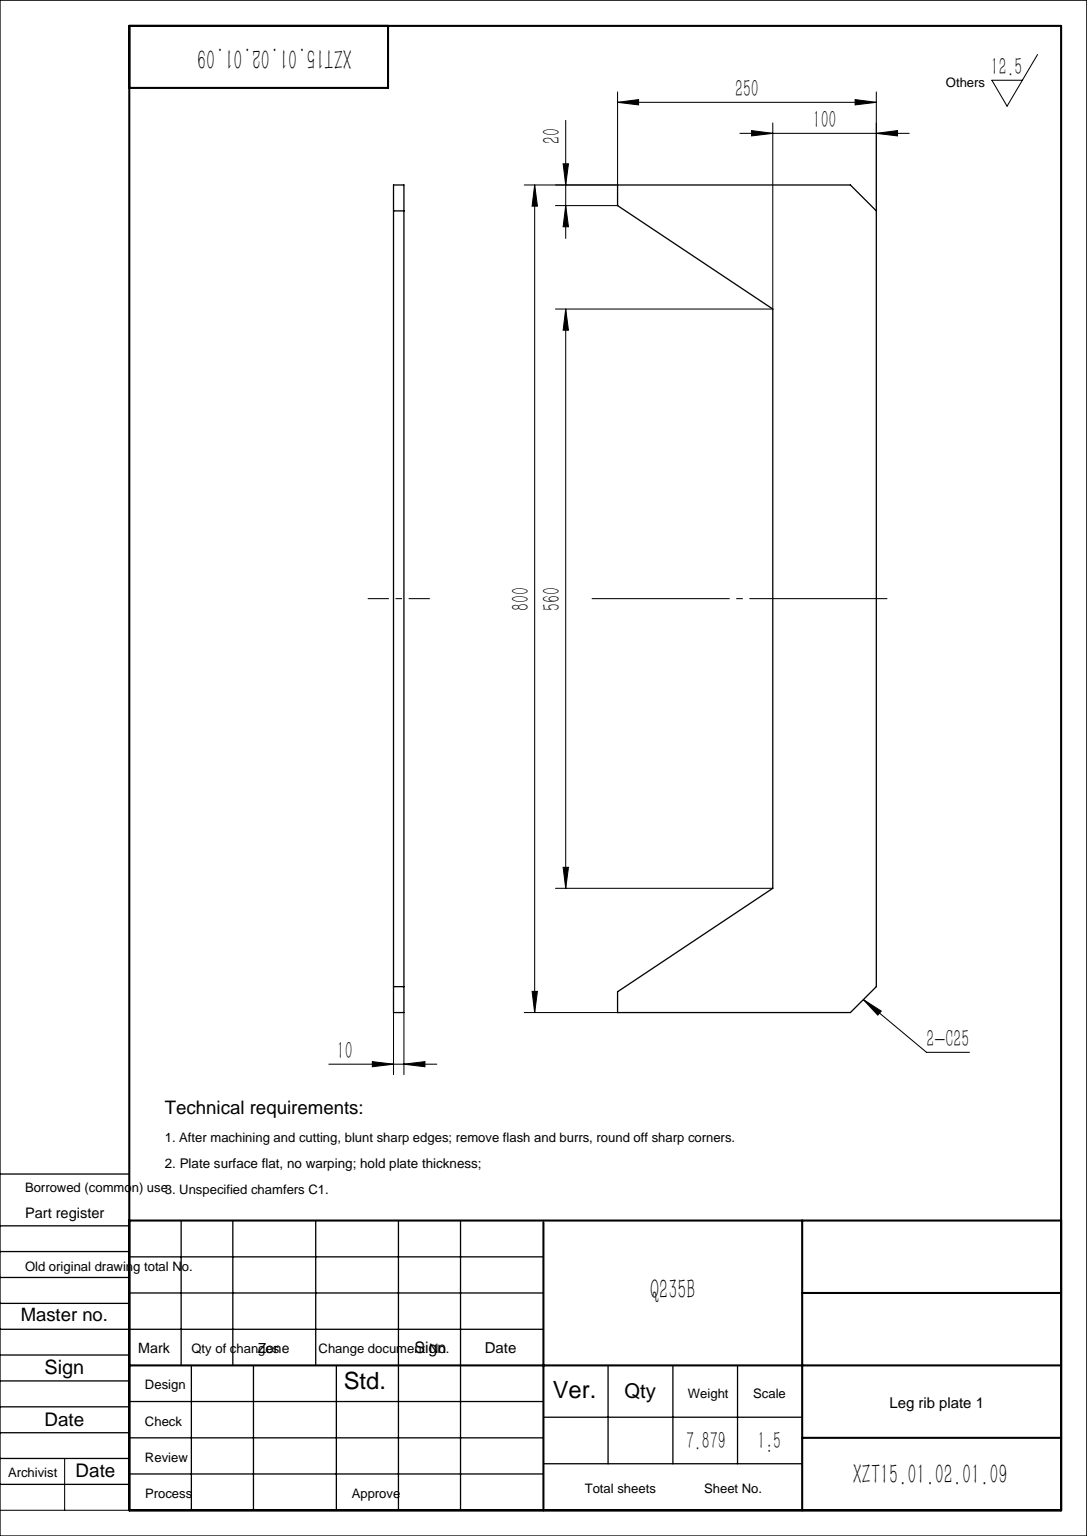
from build123d import *

# Parameters (mm, degrees)
BOSS_EXTRUDE1_DEPTH = 5
CHAMFER1_SIZE       = 25


with BuildPart() as part:
    # Sketch1 → Boss-Extrude1 (new, symmetric)
    with BuildSketch(Plane.XY):
        Polygon((0, -280), (0, 280), (-150, 380), (-150, 400), (100, 400), (100, -400), (-150, -400), (-150, -380), align=None)
    extrude(amount=BOSS_EXTRUDE1_DEPTH, both=True)

    # Chamfer1
    chamfer1_edges = [part.edges().sort_by_distance(p)[0] for p in [
        (100, 400, 0),
        (100, -400, 0),
    ]]
    chamfer(chamfer1_edges, length=CHAMFER1_SIZE)


solid = part.part
